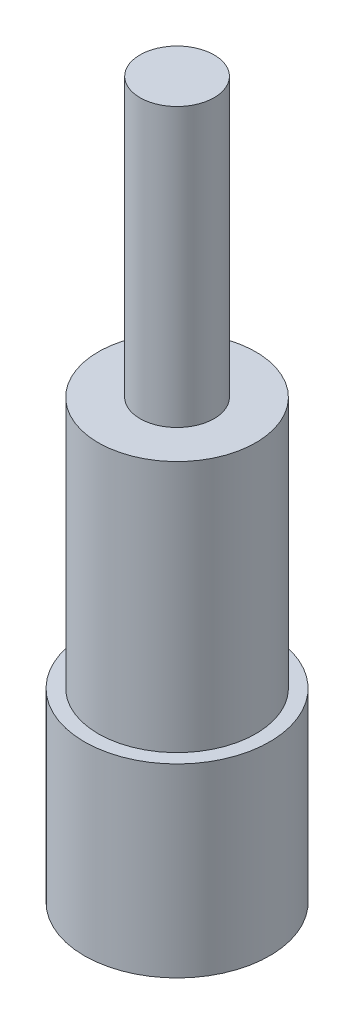
from build123d import *

# Parameters (mm, degrees)
SKETCH1_R           = 10
BOSS_EXTRUDE1_DEPTH = 20
SKETCH2_R           = 8.5
BOSS_EXTRUDE2_DEPTH = 27.2
SKETCH3_R           = 4
BOSS_EXTRUDE3_DEPTH = 30
CUT_EXTRUDE1_DEPTH  = 1.2


with BuildPart() as part:
    # Sketch1 → Boss-Extrude1 (new body)
    with BuildSketch(Plane(origin=(0, 0, 0), x_dir=(1, 0, 0), z_dir=(0, 1, 0))):
        with Locations(Location((0, 0, 0), (0, 0, 270))):
            Circle(SKETCH1_R)
    extrude(amount=BOSS_EXTRUDE1_DEPTH)

    # Sketch2 → Boss-Extrude2 (add)
    with BuildSketch(Plane(origin=(0, 20, 0), x_dir=(1, 0, 0), z_dir=(0, 1, 0))):
        with Locations(Location((0, 0, 0), (0, 0, 270))):
            Circle(SKETCH2_R)
    extrude(amount=BOSS_EXTRUDE2_DEPTH)

    # Sketch3 → Boss-Extrude3 (add)
    with BuildSketch(Plane(origin=(0, 47.2, 0), x_dir=(1, 0, 0), z_dir=(0, 1, 0))):
        with Locations(Location((0, 0, 0), (0, 0, 270))):
            Circle(SKETCH3_R)
    extrude(amount=BOSS_EXTRUDE3_DEPTH)

    # Sketch4 → Cut-Extrude1 (cut)
    with BuildSketch(Plane(origin=(0, 0, -4), x_dir=(-1, 0, 0), z_dir=(0, 0, -1))):
        with BuildLine():
            Line((-1, 50.2), (-1, 64.2))
            ThreePointArc((-1, 64.2), (0, 65.2), (1, 64.2))
            Line((1, 64.2), (1, 50.2))
            ThreePointArc((1, 50.2), (0, 49.2), (-1, 50.2))
        make_face()
    extrude(amount=-CUT_EXTRUDE1_DEPTH, mode=Mode.SUBTRACT)


solid = part.part
